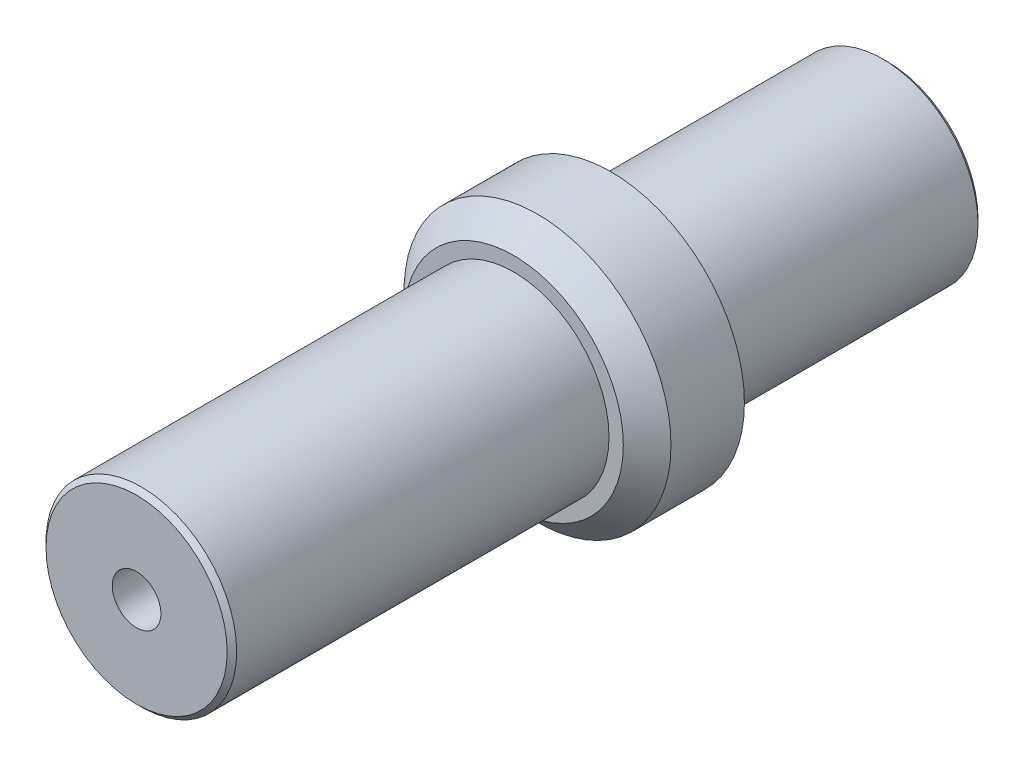
from build123d import *

# Parameters (mm, degrees)
SKETCH_1_R              = 20
EXTRUDE_1_DEPTH         = 58
SKETCH_2_R              = 28
EXTRUDE_2_DEPTH         = 20.4
SKETCH_3_R              = 20
EXTRUDE_3_DEPTH         = 79.1
CHAMFER_1_SIZE          = 5
CHAMFER_2_SIZE          = 1
HOLE_WIZARD_M12_1_D     = 10.2
HOLE_WIZARD_M12_1_DEPTH = 29.25
HOLE_WIZARD_M12_1_TIP   = 3.064389157
HOLE_WIZARD_M12_2_D     = 10.2
HOLE_WIZARD_M12_2_DEPTH = 29.25
HOLE_WIZARD_M12_2_TIP   = 3.064389157


with BuildPart() as part:
    # 草图1 → 凸台-拉伸1 (new body)
    with BuildSketch(Plane.XY):
        with Locations(Location((0, 0, 0), (0, 0, 180))):
            Circle(SKETCH_1_R)
    extrude(amount=EXTRUDE_1_DEPTH)

    # 草图2 → 凸台-拉伸2 (add)
    with BuildSketch(Plane.XY.offset(58)):
        Circle(SKETCH_2_R)
    extrude(amount=EXTRUDE_2_DEPTH)

    # 草图3 → 凸台-拉伸3 (add)
    with BuildSketch(Plane.XY.offset(78.4)):
        with Locations(Location((0, 0, 0), (0, 0, 180))):
            Circle(SKETCH_3_R)
    extrude(amount=EXTRUDE_3_DEPTH)

    # 倒角1
    chamfer_1_edges = [part.edges().sort_by_distance(p)[0] for p in [
        (-28, 0, 78.4),
    ]]
    chamfer(chamfer_1_edges, length=CHAMFER_1_SIZE)

    # 倒角2
    chamfer_2_edges = [part.edges().sort_by_distance(p)[0] for p in [
        (20, 0, 157.5),
        (20, 0, 0),
    ]]
    chamfer(chamfer_2_edges, length=CHAMFER_2_SIZE)

    # M12 螺纹孔1
    with Locations(Plane(origin=(0, 0, 0), x_dir=(-1, 0, 0), z_dir=(0, 0, -1))):
        with Locations((0, 0)):
            Hole(HOLE_WIZARD_M12_1_D / 2, depth=HOLE_WIZARD_M12_1_DEPTH)
            with Locations((0, 0, -(HOLE_WIZARD_M12_1_DEPTH + HOLE_WIZARD_M12_1_TIP / 2))):  # 118° drill point
                Cone(0, HOLE_WIZARD_M12_1_D / 2, HOLE_WIZARD_M12_1_TIP, mode=Mode.SUBTRACT)

    # M12 螺纹孔2
    with Locations(Plane.XY.offset(157.5)):
        with Locations((0, 0)):
            Hole(HOLE_WIZARD_M12_2_D / 2, depth=HOLE_WIZARD_M12_2_DEPTH)
            with Locations((0, 0, -(HOLE_WIZARD_M12_2_DEPTH + HOLE_WIZARD_M12_2_TIP / 2))):  # 118° drill point
                Cone(0, HOLE_WIZARD_M12_2_D / 2, HOLE_WIZARD_M12_2_TIP, mode=Mode.SUBTRACT)


solid = part.part
